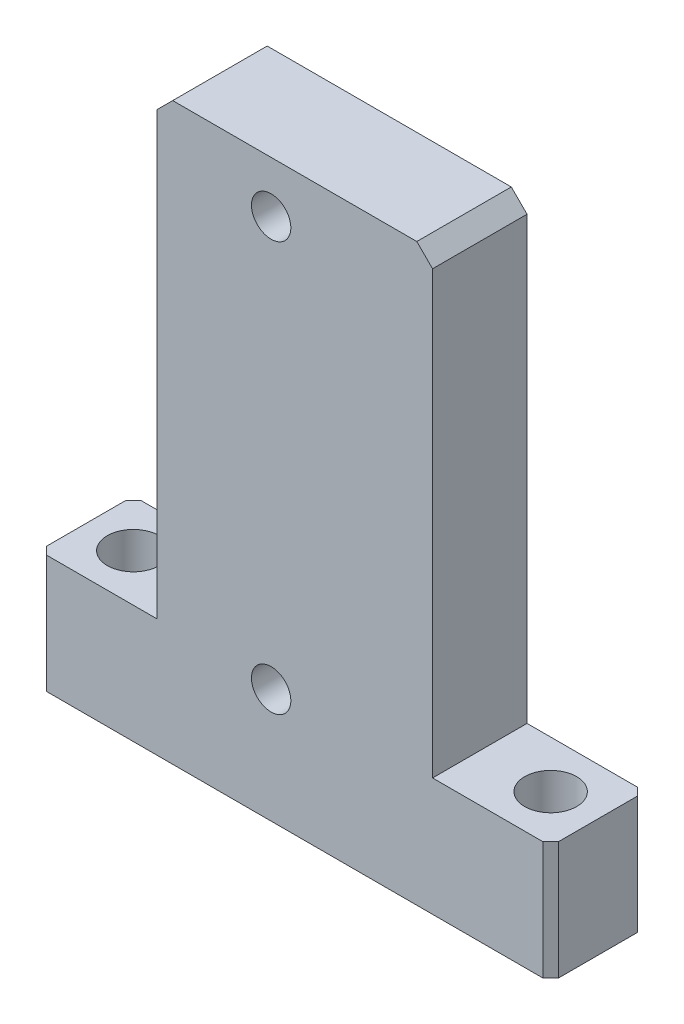
SolidWorks part; units mm, degrees
material "#45(1.1191)"
ref_plane "前视基准面" through (0, 0, 0) normal (0, 0, 1) x (1, 0, 0)
ref_plane "上视基准面" through (0, 0, 0) normal (0, 1, 0) x (1, 0, 0)
ref_plane "右视基准面" through (0, 0, 0) normal (1, 0, 0) x (0, 0, -1)
sketch "草图1" plane through (0, 0, 0) normal (0, 0, 1) x (1, 0, 0)
  line L1 (-17.5, -36.5) -> (17.5, -36.5)
  line L2 (-17.5, -36.5) -> (-17.5, 36.5)
  line L3 (-17.5, 36.5) -> (17.5, 36.5)
  line L4 (17.5, -36.5) -> (17.5, 36.5)
  line L5 (-17.5, -36.5) -> (17.5, 36.5) construction
  line L6 (-17.5, 36.5) -> (17.5, -36.5) construction
  point P0 (0, 0)
  dimension "D1" = 35
  dimension "D2" = 73
extrude "凸台-拉伸1" add sketch "草图1" along normal mid plane 12
sketch "草图2" plane through (0, -36.5, 0) normal (0, -1, 0) x (1, 0, 0)
  line L0 (-17.5, 6) -> (17.5, 6) construction
  line L1 (32.5, -6) -> (-32.5, -6)
  line L2 (32.5, -6) -> (32.5, 6)
  line L3 (32.5, 6) -> (-32.5, 6)
  line L4 (-32.5, -6) -> (-32.5, 6)
  line L5 (32.5, -6) -> (-32.5, 6) construction
  line L6 (32.5, 6) -> (-32.5, -6) construction
  point P0 (0, 0)
  dimension "D1" = 65
extrude "凸台-拉伸2" add sketch "草图2" against normal blind 15
sketch "草图3" plane through (0, -21.5, 0) normal (0, 1, 0) x (1, 0, 0)
  line L0 (-26.5, 0) -> (0, 0) construction
  line L1 (0, 0) -> (26.5, 0) construction
  line L3 (-32.5, -6) -> (-32.5, 6) construction
  point P0 (-26.5, 0)
  point P2 (26.5, 0)
  dimension "D1" = 6
hole_wizard "M6 间隙孔1" positions "草图3" profile "草图4" hole size "M6" standard "ISO" end condition through all
sketch "草图4" plane through (-26.5, -21.5, 0) normal (1, 0, 0) x (0, 0, 1)
  line L0 (0, 0) -> (0, 15)
  line L1 (0, 15) -> (3.3, 15)
  line L2 (3.3, 15) -> (3.3, 0)
  line L5 (3.3, 0) -> (0, 0)
  line L11 (0, -6.35) -> (0, 107.95) construction
  dimension "通孔孔直径" = 6.6
  dimension "通孔孔深度" = 15
sketch "草图5" plane through (0, -36.5, 0) normal (0, -1, 0) x (-1, 0, 0)
  line L0 (10, 0) -> (0, 0) construction
  line L1 (0, 0) -> (-10, 0) construction
  point P0 (10, 0)
  point P2 (-10, 0)
  dimension "D1" = 20
hole_wizard "Ø6.0mm 暗销孔1" positions "草图5" profile "草图6" hole size "Ø6.0" standard "ISO"
sketch "草图6" plane through (-10, -36.5, 0) normal (1, 0, 0) x (0, 0, -1)
  line L0 (0, 0) -> (0, 16.8026)
  line L1 (0, 16.8026) -> (3, 15)
  line L2 (3, 15) -> (3, 0)
  line L5 (3, 0) -> (0, 0)
  line L10 (0, 16.8026) -> (-3, 15) construction
  line L11 (0, -6.35) -> (0, 107.95) construction
  dimension "孔直径" = 6
  dimension "孔深度" = 15
  dimension "导头角度" = 118
sketch "草图7" plane through (0, 0, -6) normal (0, 0, -1) x (-1, 0, 0)
  point P0 (3, -22)
  point P3 (3, 30)
hole_wizard "M6 螺纹孔1" positions "草图7" profile "草图8" tap size "M6" standard "ISO" end condition through all
cosmetic thread "孔螺蚊线1" parameters "D2"=6
cosmetic thread "孔螺蚊线2" parameters "D2"=6
sketch "草图8" plane through (-3, -22, -6) normal (1, 0, 0) x (0, 1, 0)
  line L0 (0, 0) -> (0, 12)
  line L1 (0, 12) -> (2.5, 12)
  line L2 (2.5, 12) -> (2.5, 0)
  line L5 (2.5, 0) -> (0, 0)
  line L11 (0, -6.35) -> (0, 107.95) construction
  dimension "通孔螺纹孔钻头直径" = 5
  dimension "通孔螺纹孔钻头深度" = 12
chamfer "倒角1" distance 1 angle 45 4 edges at (32.5, -29, -6) (32.5, -29, 6) (-32.5, -29, 6) (-32.5, -29, -6)
chamfer "倒角2" distance 2 angle 45 2 edges at (17.5, 36.5, 0) (-17.5, 36.5, 0)
